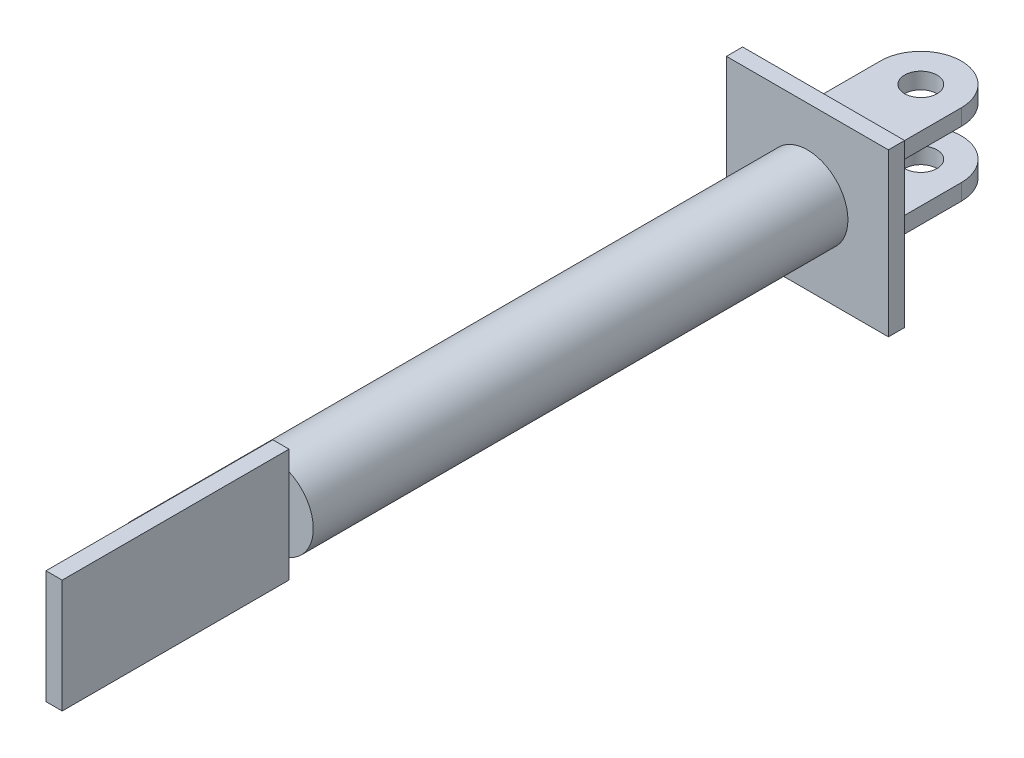
SolidWorks part; units mm, degrees
ref_plane "Front Plane" through (0, 0, 0) normal (0, 0, 1) x (1, 0, 0)
ref_plane "Top Plane" through (0, 0, 0) normal (0, 1, 0) x (1, 0, 0)
ref_plane "Right Plane" through (0, 0, 0) normal (1, 0, 0) x (0, 0, -1)
other "Configuration Table"
sketch "Sketch1" plane through (0, 0, 0) normal (0, 0, 1) x (1, 0, 0)
  line L1 (-50, 50) -> (50, 50)
  line L2 (-50, 50) -> (-50, -50)
  line L3 (-50, -50) -> (50, -50)
  line L4 (50, 50) -> (50, -50)
  line L5 (-50, 50) -> (50, -50) construction
  line L6 (-50, -50) -> (50, 50) construction
  point P0 (0, 0)
  dimension "D1" = 100
  dimension "D2" = 100
extrude "Boss-Extrude1" add sketch "Sketch1" along normal mid plane 10
sketch "Sketch2" plane through (0, 0, 0) normal (0, 1, 0) x (1, 0, 0)
  line L0 (50, 5) -> (-50, 5) construction
  line L1 (-25, 5) -> (25, 5)
  line L2 (-25, 5) -> (-25, 65)
  line L4 (25, 5) -> (25, 65)
  line L5 (-50, -5) -> (-50, 5) construction
  arc A0 (25, 65) -> (-25, 65) centre (0, 65) ccw
  circle A1 centre (0, 65) radius 10
  dimension "D4" = 20
  dimension "D1" = 50
  dimension "D2" = 25
  dimension "D3" = 60
extrude "Boss-Extrude2" add sketch "Sketch2" along normal mid plane 50
sketch "Sketch3" plane through (0, 0, -5) normal (0, 0, -1) x (-1, 0, 0)
  line L0 (-25, 25) -> (-25, -25) construction
  line L1 (-25, 15) -> (25, 15)
  line L2 (-25, 15) -> (-25, -15)
  line L3 (-25, -15) -> (25, -15)
  line L4 (25, 15) -> (25, -15)
  line L5 (25, 25) -> (25, -25) construction
  line L6 (25, 25) -> (-25, 25) construction
  line L7 (-25, -25) -> (25, -25) construction
  dimension "D1" = 10
  dimension "D2" = 10
extrude "Cut-Extrude1" cut sketch "Sketch3" along normal blind 130
sketch "Sketch4" plane through (0, 0, 5) normal (0, 0, 1) x (1, 0, 0)
  circle A0 centre (0, 0) radius 25
  dimension "D1" = 50
extrude "Boss-Extrude3" add sketch "Sketch4" along normal blind 400
sketch "Sketch5" plane through (0, 0, 405) normal (0, 0, 1) x (1, 0, 0)
  line L0 (0, 25) -> (0, -25)
  arc A0 (0, -25) -> (0, 25) centre (0, 0) ccw
extrude "Cut-Extrude2" cut sketch "Sketch5" against normal blind 70
sketch "Sketch7" plane through (0, 0, 0) normal (1, 0, 0) x (0, 0, -1)
  line L0 (-335, 25) -> (-335, -25) construction
  line L1 (-335, 35) -> (-475, 35)
  line L2 (-335, 35) -> (-335, -35)
  line L3 (-335, -35) -> (-475, -35)
  line L4 (-475, 35) -> (-475, -35)
  line L5 (-335, 25) -> (-405, 25) construction
  line L6 (-335, -25) -> (-405, -25) construction
  dimension "D1" = 140
  dimension "D2" = 10
  dimension "D3" = 10
extrude "Boss-Extrude4" add sketch "Sketch7" along normal blind 10
